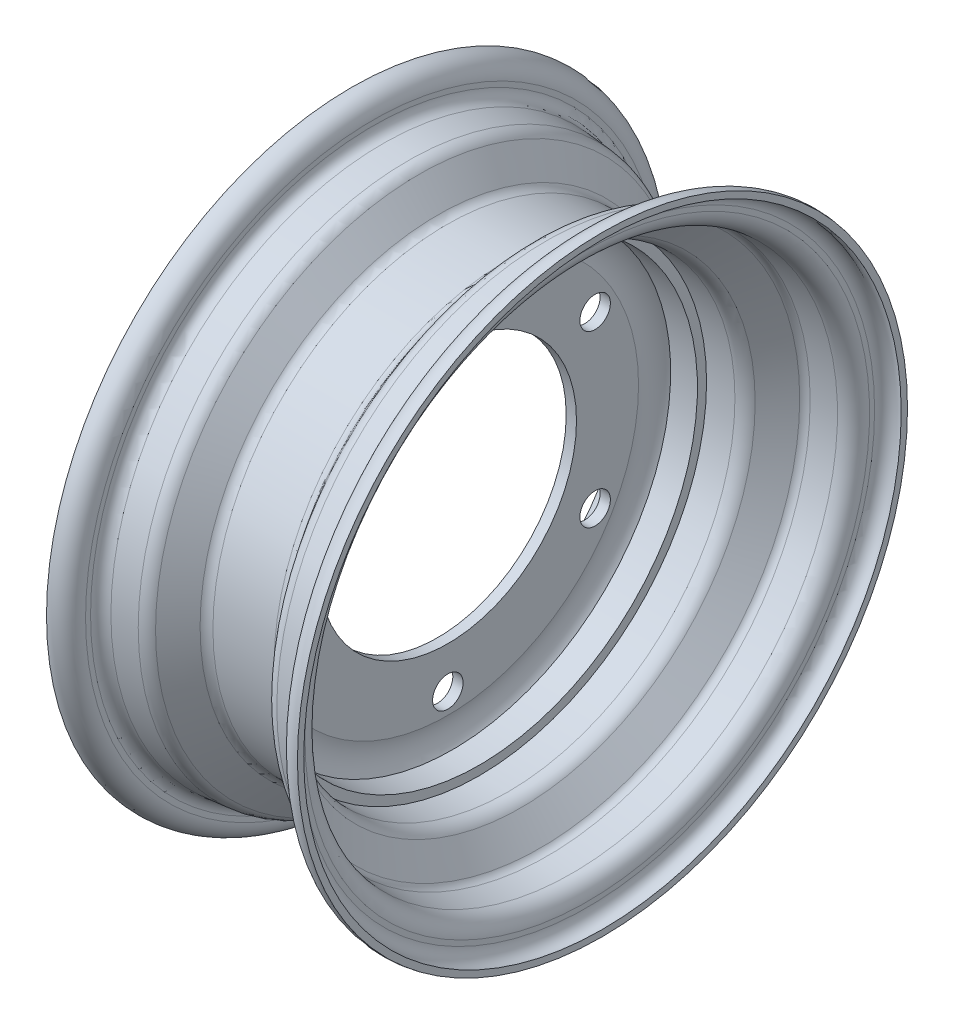
from build123d import *

# Parameters (mm, degrees)
SCALE_1_SCALE       = 0.731343284
CUT_EXTRUDE_2_REACH = 199.039
SKETCH_4_R          = 6.5


with BuildPart() as part:
    # 草图2 → 旋转1 (revolve)
    with BuildSketch(Plane.XY, mode=Mode.PRIVATE) as revolve_1_sk:
        with BuildLine():
            Line((55.03343969, 158.353580236), (40.387179575, 157.072222603))
            ThreePointArc((40.387179575, 157.072222603), (36.757353818, 155.957845796), (33.90043136, 153.456753082))
            Line((33.90043136, 153.456753082), (22.81007227, 138.595551029))
            ThreePointArc((22.81007227, 138.595551029), (20.615656314, 136.757442651), (17.830091986, 136.098098151))
            Line((17.830091986, 136.098098151), (-17.830091986, 136.098098151))
            ThreePointArc((-17.830091986, 136.098098151), (-20.615656314, 136.757442651), (-22.81007227, 138.595551029))
            Line((-22.81007227, 138.595551029), (-33.90043136, 153.456753082))
            ThreePointArc((-33.90043136, 153.456753082), (-36.757353818, 155.957845796), (-40.387179575, 157.072222603))
            Line((-40.387179575, 157.072222603), (-55.03343969, 158.353580236))
            ThreePointArc((-55.03343969, 158.353580236), (-59.073188734, 160.345757851), (-60.705705036, 164.543761485))
            Line((-60.705705036, 164.543761485), (-60.705705036, 167.453055254))
            ThreePointArc((-60.705705036, 167.453055254), (-64.495112644, 175.536358254), (-73.132352941, 177.794117647))
            Line((-73.132352941, 177.794117647), (-73.132352941, 174.115893968))
            ThreePointArc((-73.132352941, 174.115893968), (-67.050399463, 172.988692483), (-64.290424508, 167.453055254))
            Line((-64.290424508, 167.453055254), (-64.290424508, 164.543761485))
            ThreePointArc((-64.290424508, 164.543761485), (-61.716119183, 157.923954321), (-55.345862749, 154.782501193))
            Line((-55.345862749, 154.782501193), (-40.699602634, 153.501143561))
            ThreePointArc((-40.699602634, 153.501143561), (-38.50256908, 152.826641973), (-36.773352605, 151.312799441))
            Line((-36.773352605, 151.312799441), (-25.682993515, 136.451597389))
            ThreePointArc((-25.682993515, 136.451597389), (-22.223009506, 133.553284489), (-17.830936762, 132.513378715))
            ThreePointArc((-17.830936762, 132.513378715), (-23.324500539, 124.729410215), (-23.701325224, 115.209567162))
            ThreePointArc((-23.701325224, 115.209567162), (-23.176627808, 113.215866858), (-23, 111.161858362))
            Line((-23, 111.161858362), (-23, 75))
            Line((-23, 75), (-17, 75))
            Line((-17, 75), (-17, 111.161858362))
            ThreePointArc((-17, 111.161858362), (-17.531511204, 119.495717118), (-14.305208, 127.198098151))
            Line((-14.305208, 127.198098151), (1.3, 127.198098151))
            Line((1.3, 127.198098151), (1.3, 132.513378678))
            Line((1.3, 132.513378678), (17.830091986, 132.513378678))
            ThreePointArc((17.830091986, 132.513378678), (22.222631941, 133.553095131), (25.682993515, 136.451597389))
            Line((25.682993515, 136.451597389), (36.773352605, 151.312799441))
            ThreePointArc((36.773352605, 151.312799441), (38.50256908, 152.826641973), (40.699602634, 153.501143561))
            Line((40.699602634, 153.501143561), (55.345862749, 154.782501193))
            ThreePointArc((55.345862749, 154.782501193), (61.716119183, 157.923954321), (64.290424508, 164.543761485))
            Line((64.290424508, 164.543761485), (64.290424508, 167.453055254))
            ThreePointArc((64.290424508, 167.453055254), (67.050399463, 172.988692483), (73.132352941, 174.115893968))
            Line((73.132352941, 174.115893968), (73.132352941, 177.794117647))
            ThreePointArc((73.132352941, 177.794117647), (64.495112644, 175.536358254), (60.705705036, 167.453055254))
            Line((60.705705036, 167.453055254), (60.705705036, 164.543761485))
            ThreePointArc((60.705705036, 164.543761485), (59.073188734, 160.345757851), (55.03343969, 158.353580236))
        make_face()
    revolve(revolve_1_sk.sketch.rotate(Axis((0, 0, 0), (1, 0, 0)), 90), axis=Axis((0, 0, 0), (1, 0, 0)))


with BuildPart() as part_1:
    # 缩放比例1: scaled about (0, 0, 0)
    add(part.part.scale(SCALE_1_SCALE))

    # 草图4 → 切除-拉伸2 (cut, up to next)
    with BuildSketch(Plane.ZY.offset(16.820895522), mode=Mode.PRIVATE) as cut_extrude_2_sk1:
        with Locations((0, 72.5)):
            Circle(SKETCH_4_R)
    cut_extrude_2_tool1 = extrude(cut_extrude_2_sk1.sketch, amount=-CUT_EXTRUDE_2_REACH, mode=Mode.PRIVATE) & part_1.part
    # 草图4 → 切除-拉伸2 (cut, up to next)
    with BuildSketch(Plane.ZY.offset(16.820895522), mode=Mode.PRIVATE) as cut_extrude_2_sk2:
        with Locations((62.786841774, 36.25)):
            Circle(SKETCH_4_R)
    cut_extrude_2_tool2 = extrude(cut_extrude_2_sk2.sketch, amount=-CUT_EXTRUDE_2_REACH, mode=Mode.PRIVATE) & part_1.part
    # 草图4 → 切除-拉伸2 (cut, up to next)
    with BuildSketch(Plane.ZY.offset(16.820895522), mode=Mode.PRIVATE) as cut_extrude_2_sk3:
        with Locations((62.786841774, -36.25)):
            Circle(SKETCH_4_R)
    cut_extrude_2_tool3 = extrude(cut_extrude_2_sk3.sketch, amount=-CUT_EXTRUDE_2_REACH, mode=Mode.PRIVATE) & part_1.part
    # 草图4 → 切除-拉伸2 (cut, up to next)
    with BuildSketch(Plane.ZY.offset(16.820895522), mode=Mode.PRIVATE) as cut_extrude_2_sk4:
        with Locations((0, -72.5)):
            Circle(SKETCH_4_R)
    cut_extrude_2_tool4 = extrude(cut_extrude_2_sk4.sketch, amount=-CUT_EXTRUDE_2_REACH, mode=Mode.PRIVATE) & part_1.part
    # 草图4 → 切除-拉伸2 (cut, up to next)
    with BuildSketch(Plane.ZY.offset(16.820895522), mode=Mode.PRIVATE) as cut_extrude_2_sk5:
        with Locations((-62.786841774, -36.25)):
            Circle(SKETCH_4_R)
    cut_extrude_2_tool5 = extrude(cut_extrude_2_sk5.sketch, amount=-CUT_EXTRUDE_2_REACH, mode=Mode.PRIVATE) & part_1.part
    # 草图4 → 切除-拉伸2 (cut, up to next)
    with BuildSketch(Plane.ZY.offset(16.820895522), mode=Mode.PRIVATE) as cut_extrude_2_sk6:
        with Locations((-62.786841774, 36.25)):
            Circle(SKETCH_4_R)
    cut_extrude_2_tool6 = extrude(cut_extrude_2_sk6.sketch, amount=-CUT_EXTRUDE_2_REACH, mode=Mode.PRIVATE) & part_1.part
    add(cut_extrude_2_tool1.solids().sort_by_distance((-16.820896, 72.5, 0))[0], mode=Mode.SUBTRACT)
    add(cut_extrude_2_tool2.solids().sort_by_distance((-16.820896, 36.25, 62.786842))[0], mode=Mode.SUBTRACT)
    add(cut_extrude_2_tool3.solids().sort_by_distance((-16.820896, -36.25, 62.786842))[0], mode=Mode.SUBTRACT)
    add(cut_extrude_2_tool4.solids().sort_by_distance((-16.820896, -72.5, 0))[0], mode=Mode.SUBTRACT)
    add(cut_extrude_2_tool5.solids().sort_by_distance((-16.820896, -36.25, -62.786842))[0], mode=Mode.SUBTRACT)
    add(cut_extrude_2_tool6.solids().sort_by_distance((-16.820896, 36.25, -62.786842))[0], mode=Mode.SUBTRACT)


solid = part_1.part
